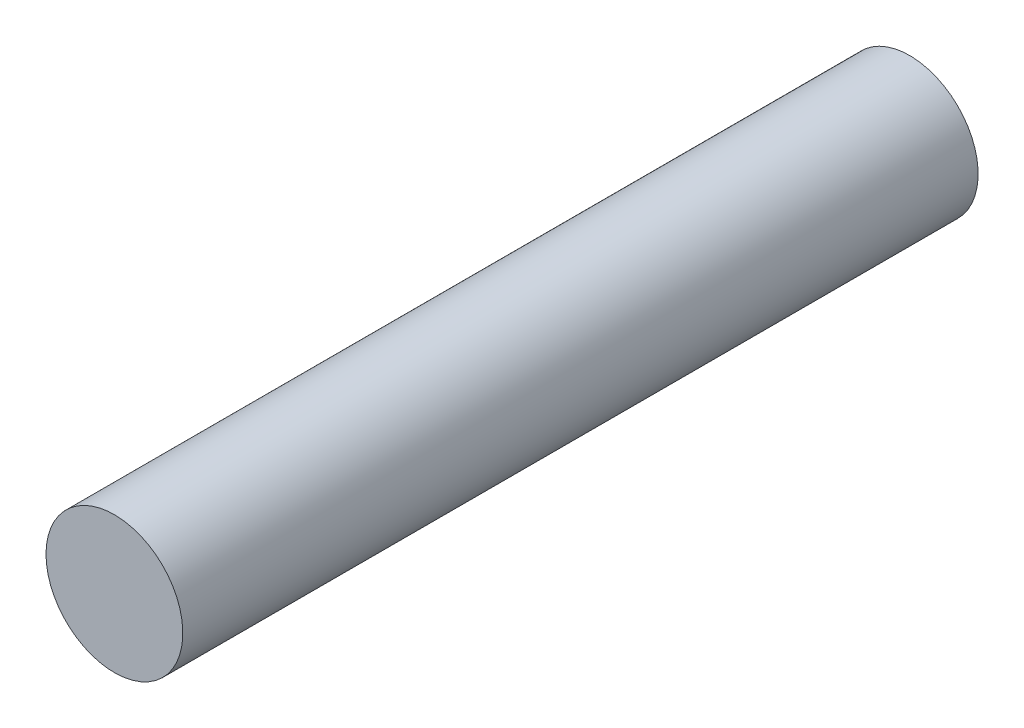
from build123d import *

# Parameters (mm, degrees)
SKETCH1_R           = 4
BOSS_EXTRUDE1_DEPTH = 46.5


with BuildPart() as part:
    # Sketch1 → Boss-Extrude1 (new body)
    with BuildSketch(Plane.XY):
        with Locations(Location((0, 0, 0), (0, 0, 180))):
            Circle(SKETCH1_R)
    extrude(amount=BOSS_EXTRUDE1_DEPTH)


solid = part.part
